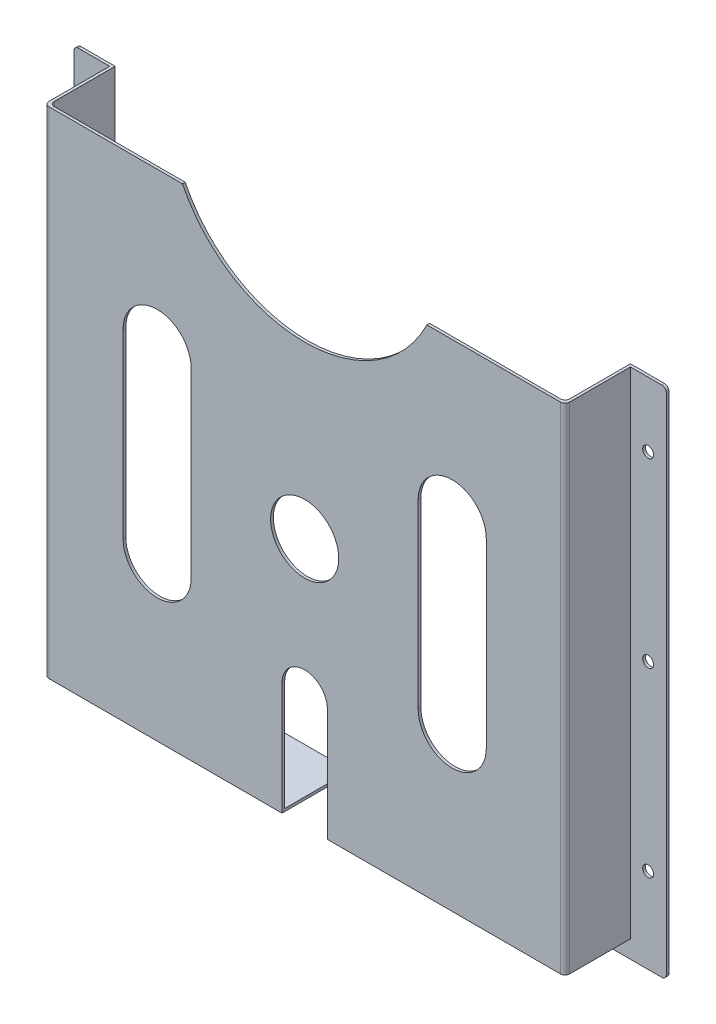
SolidWorks part; units mm, degrees
ref_plane "Front Plane" through (0, 0, 0) normal (0, 0, 1) x (1, 0, 0)
ref_plane "Top Plane" through (0, 0, 0) normal (0, 1, 0) x (1, 0, 0)
ref_plane "Right Plane" through (0, 0, 0) normal (1, 0, 0) x (0, 0, -1)
sketch "Sketch1" plane through (0, 0, 0) normal (0, 0, 1) x (1, 0, 0)
  line L1 (-113.5, 108.5) -> (113.5, 108.5)
  line L2 (-113.5, 108.5) -> (-113.5, -108.5)
  line L3 (-113.5, -108.5) -> (113.5, -108.5)
  line L4 (113.5, 108.5) -> (113.5, -108.5)
  line L5 (-113.5, 108.5) -> (113.5, -108.5) construction
  line L6 (-113.5, -108.5) -> (113.5, 108.5) construction
  point P0 (0, 0)
  dimension "D1" = 227
  dimension "D2" = 217
extrude "Boss-Extrude1" add sketch "Sketch1" along normal blind 1.2
sketch "Sketch21" plane through (0, 0, 1.2) normal (0, 0, 1) x (1, 0, 0)
  line L0 (114.7, -109.7) -> (114.7, 109.7)
  line L1 (114.7, 109.7) -> (-114.7, 109.7)
  line L2 (-114.7, 109.7) -> (-114.7, -109.7)
  line L3 (-114.7, -109.7) -> (114.7, -109.7)
  line L4 (113.5, -108.5) -> (113.5, 108.5)
  line L5 (113.5, 108.5) -> (-113.5, 108.5)
  line L6 (-113.5, 108.5) -> (-113.5, -108.5)
  line L7 (-113.5, -108.5) -> (113.5, -108.5)
  line L8 (113.5, -108.5) -> (113.5, 108.5)
  line L9 (113.5, 108.5) -> (-113.5, 108.5)
  line L10 (-113.5, 108.5) -> (-113.5, -108.5)
  line L11 (-113.5, -108.5) -> (113.5, -108.5)
  dimension "D1" = 0
  dimension "D2" = 1.2
extrude "Boss-Extrude2" add sketch "Sketch21" against normal blind 30
sketch "Sketch22" plane through (0, 0, -28.8) normal (0, 0, -1) x (-1, 0, 0)
  line L1 (-130.5, 117.5) -> (130.5, 117.5)
  line L2 (-130.5, 117.5) -> (-130.5, -117.5)
  line L3 (-130.5, -117.5) -> (130.5, -117.5)
  line L4 (130.5, 117.5) -> (130.5, -117.5)
  line L5 (-130.5, 117.5) -> (130.5, -117.5) construction
  line L6 (-130.5, -117.5) -> (130.5, 117.5) construction
  line L8 (113.5, 108.5) -> (113.5, -108.5) construction
  line L9 (113.5, -108.5) -> (-113.5, -108.5) construction
  line L10 (-113.5, -108.5) -> (-113.5, 108.5) construction
  line L11 (-113.5, 108.5) -> (113.5, 108.5) construction
  line L12 (113.5, 108.5) -> (113.5, -108.5)
  line L13 (113.5, -108.5) -> (-113.5, -108.5)
  line L14 (-113.5, -108.5) -> (-113.5, 108.5)
  line L15 (-113.5, 108.5) -> (113.5, 108.5)
  point P0 (0, 0)
  dimension "D1" = 261
  dimension "D2" = 235
extrude "Boss-Extrude3" add sketch "Sketch22" against normal blind 1.2
sketch "Sketch23" plane through (0, 117.5, 0) normal (0, 1, 0) x (1, 0, 0)
  line L0 (114.7, -1.2) -> (-114.7, -1.2) construction
  line L5 (-130.5, 28.8) -> (130.5, 28.8)
  line L6 (-130.5, 28.8) -> (-130.5, -1.2)
  line L7 (-130.5, -1.2) -> (130.5, -1.2)
  line L8 (130.5, 28.8) -> (130.5, -1.2)
extrude "Cut-Extrude1" cut sketch "Sketch23" against normal up to surface (9 mm away) up to face at (0, 108.5, -14.4)
sketch "Sketch24" plane through (0, 0, 1.2) normal (0, 0, 1) x (1, 0, 0)
  line L0 (0, 0) -> (0, 79.3095) construction
  line L1 (-65, -40) -> (-65, 40) construction
  line L2 (-80, -40) -> (-80, 40)
  line L3 (-50, -40) -> (-50, 40)
  line L4 (65, -40) -> (65, 40) construction
  line L5 (80, -40) -> (80, 40)
  line L6 (50, -40) -> (50, 40)
  line L7 (0, -60) -> (0, -120) construction
  line L8 (10, -60) -> (10, -120)
  line L9 (-10, -60) -> (-10, -120)
  circle A0 centre (0, 0) radius 15
  arc A1 (-80, -40) -> (-50, -40) centre (-65, -40) ccw
  arc A2 (-50, 40) -> (-80, 40) centre (-65, 40) ccw
  arc A3 (80, -40) -> (50, -40) centre (65, -40) cw
  arc A4 (50, 40) -> (80, 40) centre (65, 40) cw
  arc A5 (10, -60) -> (-10, -60) centre (0, -60) ccw
  arc A6 (-10, -120) -> (10, -120) centre (0, -120) ccw
  circle A7 centre (0, 135) radius 60
  point P6 (-65, 0)
  point P11 (0, -90)
  point P14 (65, 0)
  dimension "D1" = 30
  dimension "D3" = 15
  dimension "D5" = 10
  dimension "D7" = 120
  dimension "D2" = 80
  dimension "D4" = 130
  dimension "D6" = 60
  dimension "D8" = 135
  dimension "D9" = 60
extrude "Cut-Extrude2" cut sketch "Sketch24" against normal up to surface (28.8 mm away)
fillet "Fillet1" radius 2 4 edges at (113.5, 0, 0) (-113.5, 0, 0) (114.7, -0.6, 1.2) (-114.7, -0.6, 1.2)
fillet "Fillet2" radius 2 4 edges at (130.5, 108.5, -28.2) (130.5, -117.5, -28.2) (-130.5, -117.5, -28.2) (-130.5, 108.5, -28.2)
sketch "Sketch25" plane through (0, 0, -27.6) normal (0, 0, 1) x (1, 0, 0)
  line L0 (0, 0) -> (0, 143.9283) construction
  line L1 (-130.5, -115.5) -> (-130.5, 106.5) construction
  point P3 (-122.5, 80)
  point P4 (-122.5, 0)
  point P5 (-122.5, -80)
  point P11 (122.5, -80)
  point P12 (122.5, 0)
  point P13 (122.5, 80)
  dimension "D1" = 8
  dimension "D2" = 80
  dimension "D3" = 80
hole_wizard "M4 Clearance Hole1" positions "Sketch26" profile "Sketch27" hole size "M4" standard "GB" end condition through all
sketch "Sketch26" plane through (0, 0, -27.6) normal (0, 0, 1) x (1, 0, 0)
  point P0 (-122.5, 80)
sketch "Sketch27" plane through (-122.5, 80, -27.6) normal (1, 0, 0) x (0, -1, 0)
  line L0 (0, 0) -> (0, 1.2)
  line L1 (0, 1.2) -> (2.4, 1.2)
  line L2 (2.4, 1.2) -> (2.4, 0)
  line L5 (2.4, 0) -> (0, 0)
  line L11 (0, -6.35) -> (0, 107.95) construction
  dimension "通孔孔直径" = 4.8
  dimension "通孔孔深度" = 1.2
pattern_sketch "Sketch pattern1" of "M4 Clearance Hole1" driven by "Sketch25"
